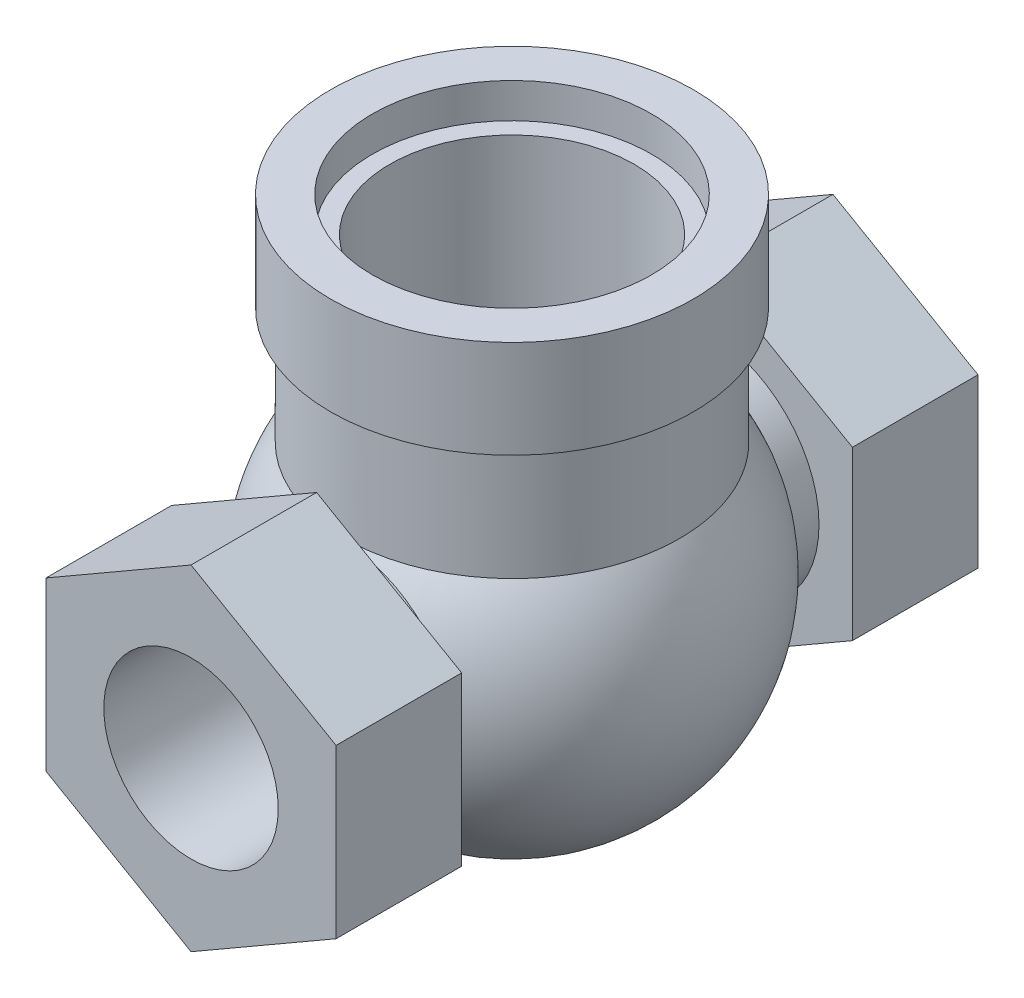
from build123d import *
from build123d.topology import SkipClean

# Parameters (mm, degrees)
SKETCH2_R           = 24
BOSS_EXTRUDE1_DEPTH = 47
SKETCH3_R           = 26
BOSS_EXTRUDE2_DEPTH = 14
SKETCH5_R           = 16
BOSS_EXTRUDE3_DEPTH = 46
BOSS_EXTRUDE4_START = 28
BOSS_EXTRUDE4_DEPTH = 18
SKETCH8_R           = 20
CUT_EXTRUDE1_DEPTH  = 5
SKETCH12_R          = 12.5
CUT_EXTRUDE3_DEPTH  = 34
CUT_EXTRUDE4_START  = -25
SKETCH13_R          = 12.5
CUT_EXTRUDE4_DEPTH  = 25
SKETCH11_R          = 17.5
CUT_EXTRUDE2_DEPTH  = 39
SKETCH16_W          = 29
SKETCH16_H          = 2.5
SKETCH17_W          = 2.5
SKETCH17_H          = 11.435558067


with BuildPart() as part:
    # Sketch1 → Revolve1 (revolve)
    with BuildSketch(Plane.XY):
        with BuildLine():
            Line((-29, 0), (29, 0))
            ThreePointArc((29, 0), (0, 29), (-29, 0))
        make_face()
    revolve(axis=Axis((-1000, 0, 0), (1, 0, 0)))

    # Sketch2 → Boss-Extrude1 (add)
    with BuildSketch(Plane(origin=(0, 0, 0), x_dir=(1, 0, 0), z_dir=(0, 1, 0))):
        with Locations(Location((0, 0, 0), (0, 0, 90))):
            Circle(SKETCH2_R)
    extrude(amount=BOSS_EXTRUDE1_DEPTH)

    # Sketch3 → Boss-Extrude2 (add)
    with BuildSketch(Plane(origin=(0, 47, 0), x_dir=(1, 0, 0), z_dir=(0, 1, 0))):
        with Locations(Location((0, 0, 0), (0, 0, 270))):
            Circle(SKETCH3_R)
    extrude(amount=-BOSS_EXTRUDE2_DEPTH)

    # Sketch5 → Boss-Extrude3 (add)
    with BuildSketch(Plane.XY):
        with Locations(Location((0, 0, 0), (0, 0, 180))):
            Circle(SKETCH5_R)
    boss_extrude3 = extrude(amount=BOSS_EXTRUDE3_DEPTH)

    # Sketch4 → Boss-Extrude4 (add)
    with BuildSketch(Plane.XY.offset(BOSS_EXTRUDE4_START)):
        Polygon((20.784609691, 12), (0, 24), (-20.784609691, 12), (-20.784609691, -12), (0, -24), (20.784609691, -12), align=None)
    boss_extrude4 = extrude(amount=BOSS_EXTRUDE4_DEPTH)

    # Sketch8 → Cut-Extrude1 (cut)
    with BuildSketch(Plane(origin=(0, 47, 0), x_dir=(1, 0, 0), z_dir=(0, 1, 0))):
        with Locations(Location((0, 0, 0), (0, 0, 270))):
            Circle(SKETCH8_R)
    extrude(amount=-CUT_EXTRUDE1_DEPTH, mode=Mode.SUBTRACT)

    # Sketch12 → Cut-Extrude3 (cut)
    with BuildSketch(Plane.XY.offset(46)):
        Circle(SKETCH12_R)
    extrude(amount=-CUT_EXTRUDE3_DEPTH, mode=Mode.SUBTRACT)

    # Mirror1: Boss-Extrude3, Boss-Extrude4 across plane
    add(boss_extrude3.mirror(Plane.XY))
    add(boss_extrude4.mirror(Plane.XY))

    # Sketch13 → Cut-Extrude4 (cut)
    with BuildSketch(Plane(origin=(0, 0, -46), x_dir=(-1, 0, 0), z_dir=(0, 0, -1)).offset(CUT_EXTRUDE4_START)):
        with Locations(Location((0, 0, 0), (0, 0, 180))):
            Circle(SKETCH13_R)
    extrude(amount=CUT_EXTRUDE4_DEPTH, mode=Mode.SUBTRACT)

    # Sketch11 → Cut-Extrude2 (cut)
    with BuildSketch(Plane(origin=(0, 42, 0), x_dir=(1, 0, 0), z_dir=(0, 1, 0))):
        with Locations(Location((0, 0, 0), (0, 0, 270))):
            Circle(SKETCH11_R)
    extrude(amount=-CUT_EXTRUDE2_DEPTH, mode=Mode.SUBTRACT)

    # Sketch15 → Cut-Revolve1 (revolve, cut)
    with BuildSketch(Plane(origin=(0, 0, 0), x_dir=(0, 0, -1), z_dir=(1, 0, 0))):
        Polygon((-6.5, 3), (0, -3.5), (0, 11), (-6.5, 11), align=None)
    revolve(axis=Axis((0, -1000, 0), (0, 1, 0)), mode=Mode.SUBTRACT)

    # Sketch16 → Cut-Revolve2 (revolve, cut)
    with BuildSketch(Plane(origin=(0, 0, 0), x_dir=(0, 0, -1), z_dir=(1, 0, 0)), mode=Mode.PRIVATE) as cut_revolve2_sk:
        with Locations((12, -6.25)):
            Rectangle(SKETCH16_W, SKETCH16_H)
    revolve(cut_revolve2_sk.sketch.rotate(Axis((0, -5, 4.897022233), (0, 0, -1)), 270), axis=Axis((0, -5, 4.897022233), (0, 0, -1)), mode=Mode.SUBTRACT)

    # Sketch17 → Cut-Revolve3 (revolve, cut)
    with SkipClean():  # the faces are left unmerged after this step: merging them gives an invalid solid
        with BuildSketch(Plane(origin=(0, 0, 0), x_dir=(0, 0, -1), z_dir=(1, 0, 0))):
            with Locations((-1.25, 0.717779034)):
                Rectangle(SKETCH17_W, SKETCH17_H)
        revolve(axis=Axis((0, -5, 0), (0, 1, 0)), mode=Mode.SUBTRACT)


solid = part.part
